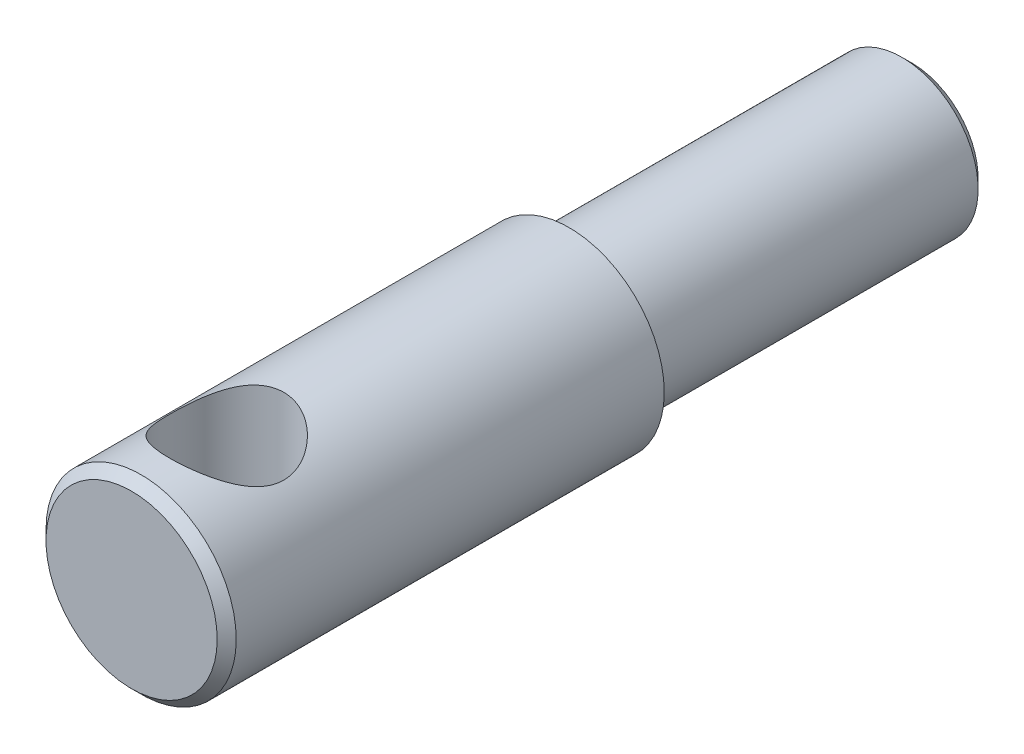
from build123d import *

# Parameters (mm, degrees)
SKETCH1_R               = 5
BOSS_EXTRUDE1_DEPTH     = 23
SKETCH2_R               = 4
BOSS_EXTRUDE2_DEPTH     = 18
CHAMFER1_SIZE           = 0.5
CUT_EXTRUDE1_DEPTH      = 25.062418831
CUT_EXTRUDE1_DEPTH_BACK = 25.062418831
SKETCH3_R               = 3


with BuildPart() as part:
    # Sketch1 → Boss-Extrude1 (new body)
    with BuildSketch(Plane.XY):
        Circle(SKETCH1_R)
    extrude(amount=BOSS_EXTRUDE1_DEPTH)

    # Sketch2 → Boss-Extrude2 (add)
    with BuildSketch(Plane(origin=(0, 0, 0), x_dir=(-1, 0, 0), z_dir=(0, 0, -1))):
        Circle(SKETCH2_R)
    extrude(amount=BOSS_EXTRUDE2_DEPTH)

    # Chamfer1
    chamfer1_edges = [part.edges().sort_by_distance(p)[0] for p in [
        (-5, 0, 23),
        (4, 0, -18),
    ]]
    chamfer(chamfer1_edges, length=CHAMFER1_SIZE)

    # Sketch3 → Cut-Extrude1 (cut, two sides: drawn at the far end of the back side and taken through both)
    with BuildSketch(Plane(origin=(0, 0, 0), x_dir=(1, 0, 0), z_dir=(0, 1, 0)).offset(-CUT_EXTRUDE1_DEPTH_BACK)):
        with Locations(Location((0, -18, 0), (0, 0, 270))):
            Circle(SKETCH3_R)
    extrude(amount=CUT_EXTRUDE1_DEPTH + CUT_EXTRUDE1_DEPTH_BACK, mode=Mode.SUBTRACT)


solid = part.part
